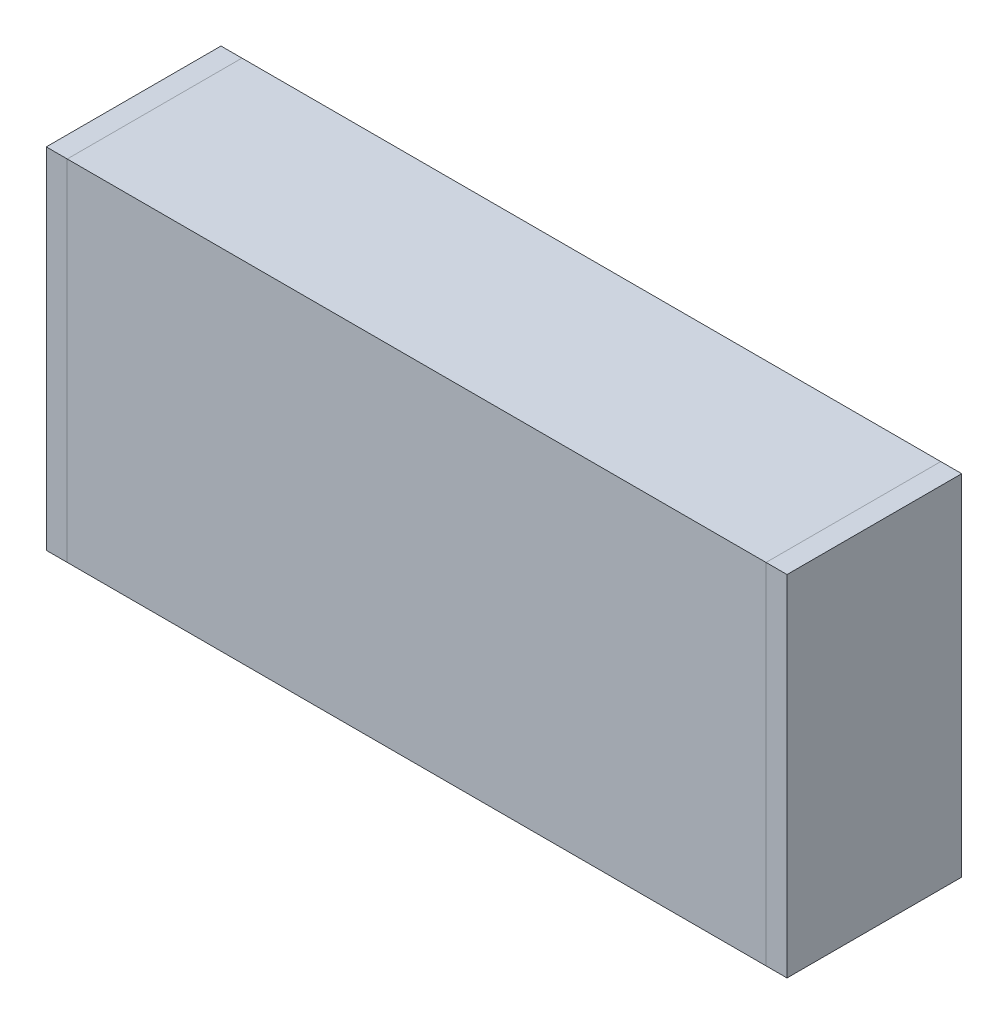
SolidWorks part; units mm, degrees
ref_plane "Front Plane" through (0, 0, 0) normal (0, 0, 1) x (1, 0, 0)
ref_plane "Top Plane" through (0, 0, 0) normal (0, 1, 0) x (1, 0, 0)
ref_plane "Right Plane" through (0, 0, 0) normal (1, 0, 0) x (0, 0, -1)
sketch3d "3DSketch1"
  line L0 (0, 0, 0) -> (200, 0, 0)
  dimension "D1" = 200
other "C-channel C80X40X15X1.5(1)"
ref_plane "Plane1" through (0, 0, 0) normal (1, 0, 0) x (0, 0, -1)
sketch "Sketch11" plane through (0, 0, 0) normal (1, 0, 0) x (0, 0, -1)
  line L0 (0, -50) -> (0, 50)
  line L1 (0, 50) -> (50, 50)
  line L2 (0, -50) -> (50, -50)
  line L3 (50, 50) -> (50, 35)
  line L4 (50, -50) -> (50, -35)
  line L5 (50, 35) -> (48.5, 35)
  line L6 (48.5, 35) -> (48.5, 48.5)
  line L7 (48.5, 48.5) -> (1.5, 48.5)
  line L8 (1.5, 48.5) -> (1.5, -48.5)
  line L9 (1.5, -48.5) -> (48.5, -48.5)
  line L10 (48.5, -48.5) -> (48.5, -35)
  line L11 (48.5, -35) -> (50, -35)
  point P2 (0, 0)
sketch "Sketch12" plane through (200, 0, 0) normal (1, 0, 0) x (0, 0, -1)
  line L1 (0, 50) -> (50, 50)
  line L2 (0, 50) -> (0, -50)
  line L3 (0, -50) -> (50, -50)
  line L4 (50, 50) -> (50, -50)
extrude "Boss-Extrude1" add sketch "Sketch12" along normal blind 6 separate body
sketch "Sketch13" plane through (0, 0, 0) normal (-1, 0, 0) x (0, 0, 1)
  line L1 (-50, 50) -> (0, 50)
  line L2 (-50, 50) -> (-50, -50)
  line L3 (-50, -50) -> (0, -50)
  line L4 (0, 50) -> (0, -50)
extrude "Boss-Extrude2" add sketch "Sketch13" along normal blind 6 separate body
sketch "Sketch14" plane through (-6, 0, 0) normal (-1, 0, 0) x (0, 0, 1)
  line L0 (-50, 0) -> (-35, 0) construction
  line L1 (-50, 50) -> (-50, -50) construction
  circle A0 centre (-35, 0) radius 6
  dimension "D1" = 12
  dimension "D2" = 15
extrude "Cut-Extrude1" cut sketch "Sketch14" against normal blind 14
equation "\"D5@Sketch11\" =\"D4@Sketch11\""
equation "\"D6@Sketch11\" =\"D4@Sketch11\""
equation "\"D7@Sketch11\" =\"D4@Sketch11\""
